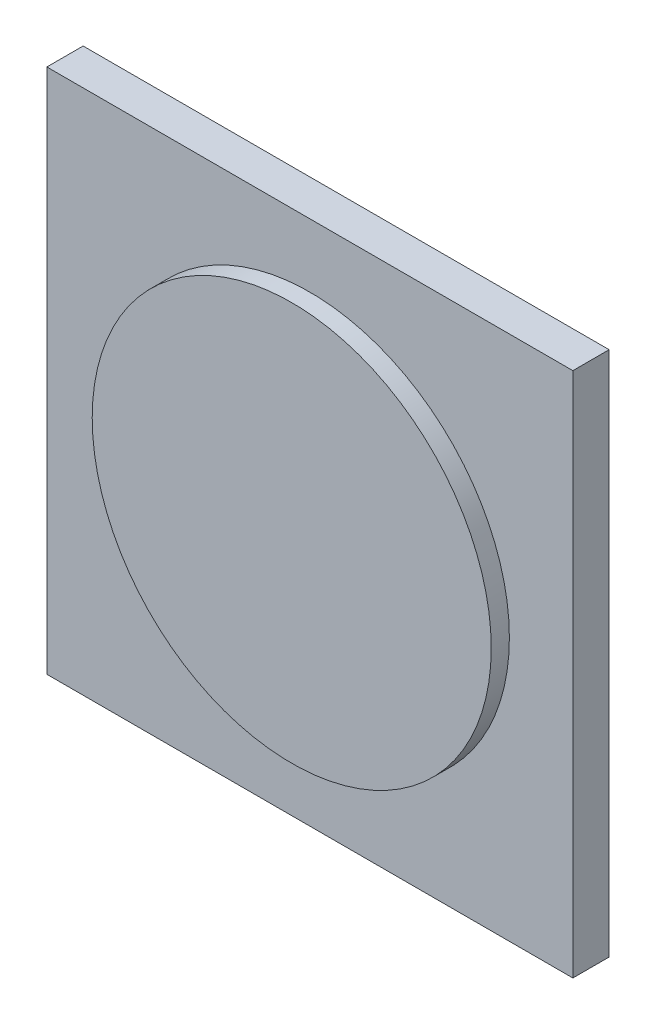
SolidWorks part; units mm, degrees
material "普通碳钢"
ref_plane "Front Plane" through (0, 0, 0) normal (0, 0, 1) x (1, 0, 0)
ref_plane "Top Plane" through (0, 0, 0) normal (0, 1, 0) x (1, 0, 0)
ref_plane "Right Plane" through (0, 0, 0) normal (1, 0, 0) x (0, 0, -1)
sketch "Sketch1" plane through (0, 0, 0) normal (0, 0, 1) x (1, 0, 0)
  line L0 (0, 0) -> (145, 0)
  line L1 (0, 0) -> (0, 145)
  line L2 (0, 145) -> (145, 145)
  line L3 (145, 145) -> (145, 0)
  dimension "D1" = 145
  dimension "D2" = 145
extrude "Boss-Extrude1" add sketch "Sketch1" along normal blind 10
sketch "Sketch2" plane through (0, 0, 10) normal (0, 0, 1) x (1, 0, 0)
  line L0 (0, 72.5) -> (145, 72.5) construction
  line L1 (0, 145) -> (0, 0) construction
  line L2 (145, 0) -> (145, 145) construction
  circle A0 centre (72.5, 72.5) radius 55
  dimension "D1" = 110
extrude "Boss-Extrude2" add sketch "Sketch2" along normal blind 5
